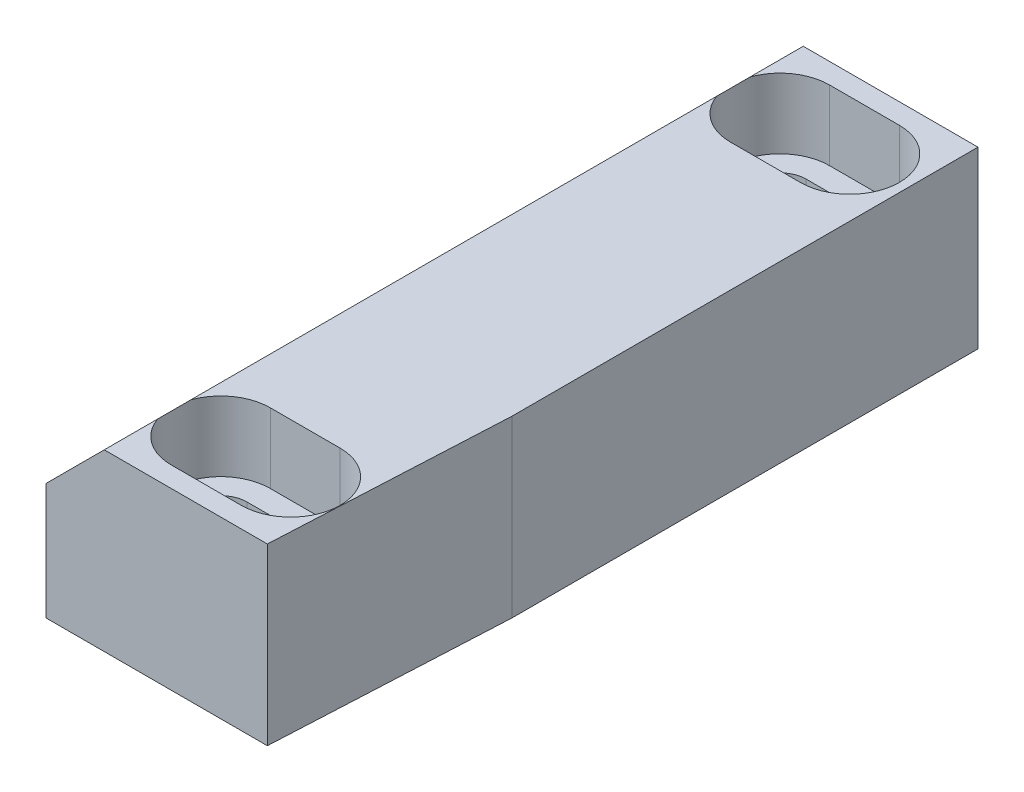
SolidWorks part; units mm, degrees
ref_plane "Front Plane" through (0, 0, 0) normal (0, 0, 1) x (1, 0, 0)
ref_plane "Top Plane" through (0, 0, 0) normal (0, 1, 0) x (1, 0, 0)
ref_plane "Right Plane" through (0, 0, 0) normal (1, 0, 0) x (0, 0, -1)
sketch "Sketch1" plane through (0, 0, 0) normal (0, 1, 0) x (1, 0, 0)
  line L1 (-10, 30) -> (10, 30)
  line L2 (-10, 30) -> (-10, -30)
  line L3 (-10, -30) -> (10, -30)
  line L4 (10, 30) -> (10, -30)
  line L5 (-10, 30) -> (10, -30) construction
  line L6 (-10, -30) -> (10, 30) construction
  point P0 (0, 0)
  dimension "D1" = 20
  dimension "D2" = 60
extrude "Boss-Extrude1" add sketch "Sketch1" along normal blind 15
chamfer "Chamfer1" distance 5 angle 45 1 edges at (-10, 15, 0)
sketch "Sketch2" plane through (0, 15, 0) normal (0, 1, 0) x (1, 0, 0)
  line L0 (10, -30) -> (9, -30)
  line L1 (-5, -30) -> (10, -30) construction
  line L2 (9, -30) -> (10, -10)
  line L3 (10, -30) -> (10, 30) construction
  line L4 (10, -10) -> (10, -30)
  dimension "D1" = 1
  dimension "D2" = 20
extrude "Cut-Extrude1" cut sketch "Sketch2" against normal through all
sketch "Sketch3" plane through (0, 15, 0) normal (0, 1, 0) x (1, 0, 0)
  line L0 (5, 24) -> (-1, 24) construction
  line L1 (5, 21.75) -> (-1, 21.75)
  line L2 (5, 26.25) -> (-1, 26.25)
  line L3 (10, -10) -> (10, 30) construction
  line L4 (10, 30) -> (-5, 30) construction
  arc A0 (5, 21.75) -> (5, 26.25) centre (5, 24) ccw
  arc A1 (-1, 26.25) -> (-1, 21.75) centre (-1, 24) ccw
  point P2 (2, 24)
  dimension "D1" = 4.5
  dimension "D2" = 8
  dimension "D3" = 6
  dimension "D4" = 6
extrude "Cut-Extrude2" cut sketch "Sketch3" against normal through all
sketch "Sketch4" plane through (0, 15, 0) normal (0, 1, 0) x (1, 0, 0)
  line L4 (-1, 19.75) -> (5, 19.75)
  line L5 (5, 28.25) -> (-1, 28.25)
  line L6 (-1, 19.75) -> (5, 19.75)
  line L7 (5, 28.25) -> (-1, 28.25)
  arc A4 (-1, 28.25) -> (-1, 19.75) centre (-1, 24) ccw
  arc A5 (5, 19.75) -> (5, 28.25) centre (5, 24) ccw
  arc A6 (-1, 28.25) -> (-1, 19.75) centre (-1, 24) ccw
  arc A7 (5, 19.75) -> (5, 28.25) centre (5, 24) ccw
  dimension "D1" = 2
extrude "Cut-Extrude3" cut sketch "Sketch4" against normal blind 6
mirror "Mirror1" about plane through (0, 0, 0) normal (0, 0, 1) of "Cut-Extrude2", "Cut-Extrude3"
